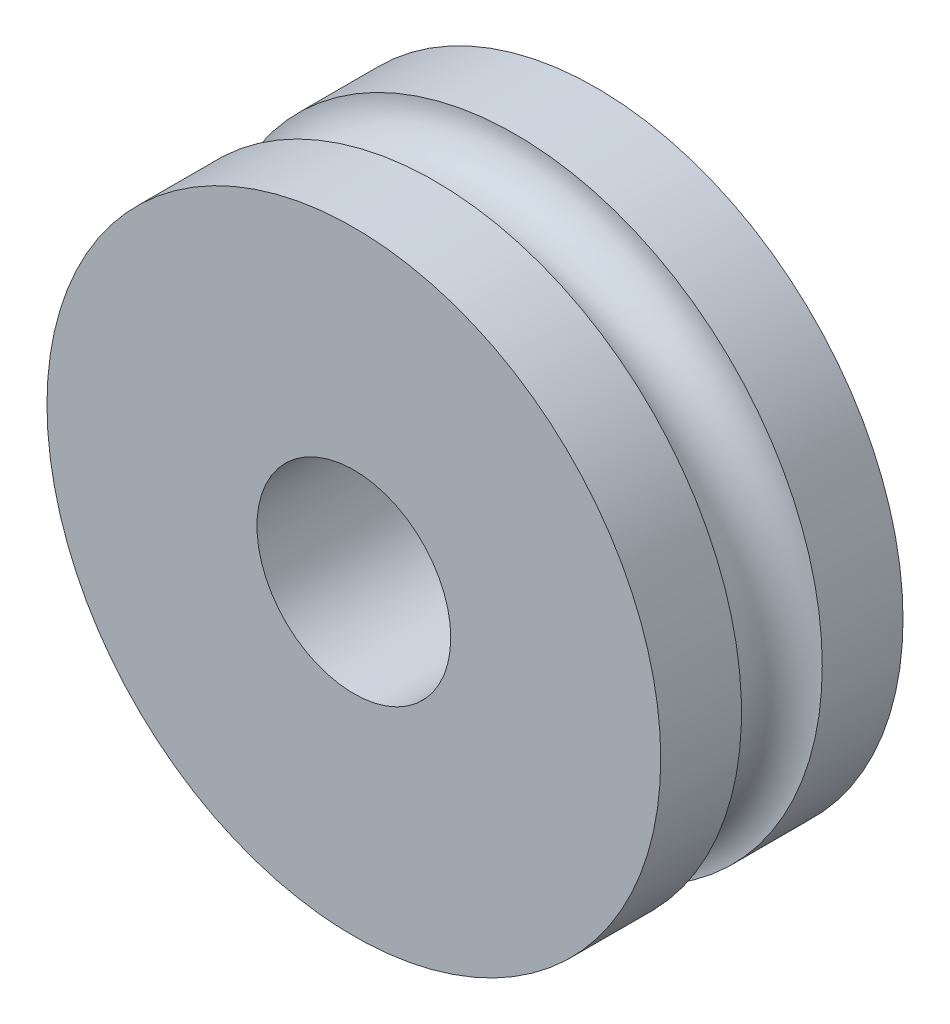
SolidWorks part; units mm, degrees
ref_plane "Front Plane" through (0, 0, 0) normal (0, 0, 1) x (1, 0, 0)
ref_plane "Top Plane" through (0, 0, 0) normal (0, 1, 0) x (1, 0, 0)
ref_plane "Right Plane" through (0, 0, 0) normal (1, 0, 0) x (0, 0, -1)
other "Configuration Table"
sketch "Sketch1" plane through (0, 0, 0) normal (0, 0, 1) x (1, 0, 0)
  circle A0 centre (0, 0) radius 38
  circle A1 centre (0, 0) radius 12
  dimension "D1" = 76
  dimension "D2" = 24
extrude "Boss-Extrude1" add sketch "Sketch1" along normal blind 30
sketch "Sketch2" plane through (0, 0, 0) normal (0, 1, 0) x (1, 0, 0)
  line L0 (-38, 0) -> (-38, -30) construction
  line L1 (0, 0) -> (0, -30)
  line L2 (-38, -30) -> (38, -30) construction
  circle A0 centre (-38, -15) radius 5
  dimension "D1" = 10
revolve "Cut-Revolve1" cut sketch "Sketch2" angle 360 about L1
